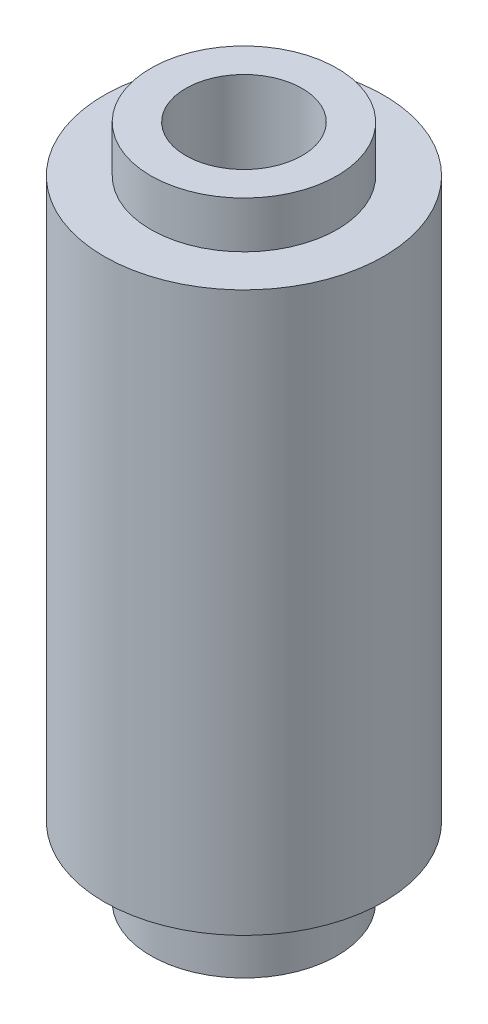
SolidWorks part; units mm, degrees
ref_plane "Front plane" through (0, 0, 0) normal (0, 0, 1) x (1, 0, 0)
ref_plane "Top plane" through (0, 0, 0) normal (0, 1, 0) x (1, 0, 0)
ref_plane "Right plane" through (0, 0, 0) normal (1, 0, 0) x (0, 0, -1)
other "Configuration Table"
sketch "Sketch 2" plane through (0, 0, 0) normal (0, 1, 0) x (1, 0, 0)
  circle A0 centre (0, 0) radius 3
  dimension "D1" = 6
extrude "Boss-Extrude 1" add sketch "Sketch 2" along normal blind 12
sketch "Sketch 3" plane through (0, 12, 0) normal (0, 1, 0) x (1, 0, 0)
  circle A0 centre (0, 0) radius 2
  dimension "D1" = 4
extrude "Boss-Extrude 2" add sketch "Sketch 3" along normal blind 1
sketch "Sketch 4" plane through (0, 0, 0) normal (0, -1, 0) x (-1, 0, 0)
  circle A0 centre (0, 0) radius 2
extrude "Boss-Extrude 3" add sketch "Sketch 4" along normal blind 1.5
sketch "Sketch 5" plane through (0, 13, 0) normal (0, 1, 0) x (1, 0, 0)
  circle A0 centre (0, 0) radius 1.25
  dimension "D1" = 2.5
extrude "Cut-Extrude 1" cut sketch "Sketch 5" against normal blind 6
sketch "Sketch 6" plane through (0, 7, 0) normal (0, 1, 0) x (1, 0, 0)
  circle A0 centre (0, 0) radius 1.5
  dimension "D1" = 3
extrude "Cut-Extrude 2" cut sketch "Sketch 6" against normal blind 2.5
sketch "Sketch 7" plane through (0, -1.5, 0) normal (0, -1, 0) x (-1, 0, 0)
  line L16 (-0.9741, 1.1407) -> (-1.3859, -0.5739)
  line L17 (-1.3859, -0.5739) -> (0.1176, -1.4954)
  line L18 (0.1176, -1.4954) -> (1.4585, -0.3503)
  line L19 (1.4585, -0.3503) -> (0.7839, 1.2789)
  line L20 (0.7839, 1.2789) -> (-0.9741, 1.1407)
  circle A0 centre (0, 0) radius 1.5 construction
  dimension "D1" = 3
extrude "Cut-Extrude 3" cut sketch "Sketch 7" against normal blind 6
